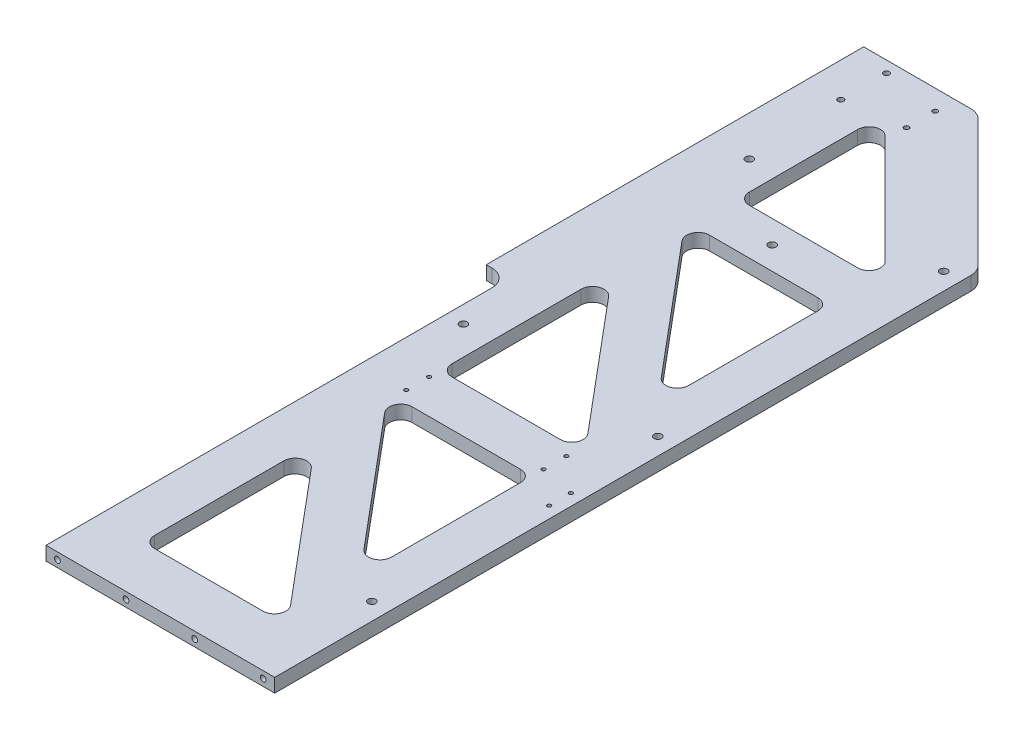
from build123d import *

# Parameters (mm, degrees)
SKETCH_1_W             = 220
SKETCH_1_H             = 330
EXTRUDE_1_DEPTH        = 6
SKETCH_2_W             = 200
SKETCH_2_H             = 405
EXTRUDE_2_DEPTH        = 12
CHAMFER_1_SIZE         = 120
FILLET_2_R             = 15
CUT_EXTRUDE_3_DEPTH    = 12
HOLE_WIZARD_M6_1_D     = 5
HOLE_WIZARD_M6_1_DEPTH = 17
HOLE_WIZARD_M6_1_TIP   = 1.502151548
HOLE_WIZARD_M6_2_D     = 5
HOLE_WIZARD_M6_2_DEPTH = 17
HOLE_WIZARD_M6_2_TIP   = 1.502151548
HOLE_WIZARD_M6_1_2_D   = 6.6
HOLE_WIZARD_M6_2_2_D   = 6.6
HOLE_WIZARD_M6_3_D     = 5
HOLE_WIZARD_M5_1_D     = 4.2
HOLE_WIZARD_M4_1_D     = 3.3
HOLE_WIZARD_M4_2_D     = 3.3


with BuildPart() as part:
    # 草图1 → 凸台-拉伸1 (new, symmetric)
    with BuildSketch(Plane(origin=(0, 0, 0), x_dir=(1, 0, 0), z_dir=(0, 1, 0))):
        Rectangle(SKETCH_1_W, SKETCH_1_H)
    extrude(amount=EXTRUDE_1_DEPTH, both=True)

    # 草图2 → 凸台-拉伸2 (add)
    with BuildSketch(Plane(origin=(0, 6, 0), x_dir=(1, 0, 0), z_dir=(0, 1, 0))):
        with Locations((10, -367.5)):
            Rectangle(SKETCH_2_W, SKETCH_2_H)
    extrude(amount=-EXTRUDE_2_DEPTH)

    # 倒角1
    chamfer_1_edges = [part.edges().sort_by_distance(p)[0] for p in [
        (110, 0, -165),
    ]]
    chamfer(chamfer_1_edges, length=CHAMFER_1_SIZE)

    # 圆角2
    fillet_2_edges = [part.edges().sort_by_distance(p)[0] for p in [
        (-10, 0, -165),
        (110, 0, -45),
        (-90, 0, 165),
    ]]
    fillet(fillet_2_edges, radius=FILLET_2_R)

    # 草图7 → 切除-拉伸3 (cut)
    with BuildSketch(Plane(origin=(0, 6, 0), x_dir=(1, 0, 0), z_dir=(0, 1, 0))):
        with BuildLine():
            Line((-34.747744438, -45), (60, -45))
            ThreePointArc((60, -45), (67.071067812, -47.928932188), (70, -55))
            Line((70, -55), (70, -167.915964824))
            ThreePointArc((70, -167.915964824), (63.420201433, -177.312891032), (52.339555569, -174.343840921))
            Line((52.339555569, -174.343840921), (-42.408188869, -61.427876097))
            ThreePointArc((-42.408188869, -61.427876097), (-43.810822308, -50.773817383), (-34.747744438, -45))
        make_face()
        with BuildLine():
            Line((-32.339555569, -135.656159079), (62.408188869, -248.572123903))
            ThreePointArc((62.408188869, -248.572123903), (63.810822308, -259.226182617), (54.747744438, -265))
            Line((54.747744438, -265), (-40, -265))
            ThreePointArc((-40, -265), (-47.071067812, -262.071067812), (-50, -255))
            Line((-50, -255), (-50, -142.084035176))
            ThreePointArc((-50, -142.084035176), (-43.420201433, -132.687108968), (-32.339555569, -135.656159079))
        make_face()
        with BuildLine():
            Line((-34.747744438, -305), (60, -305))
            ThreePointArc((60, -305), (67.071067812, -307.928932188), (70, -315))
            Line((70, -315), (70, -427.915964824))
            ThreePointArc((70, -427.915964824), (63.420201433, -437.312891032), (52.339555569, -434.343840921))
            Line((52.339555569, -434.343840921), (-42.408188869, -321.427876097))
            ThreePointArc((-42.408188869, -321.427876097), (-43.810822308, -310.773817383), (-34.747744438, -305))
        make_face()
        with BuildLine():
            Line((-32.339555569, -395.656159079), (62.408188869, -508.572123903))
            ThreePointArc((62.408188869, -508.572123903), (63.810822308, -519.226182617), (54.747744438, -525))
            Line((54.747744438, -525), (-40, -525))
            ThreePointArc((-40, -525), (-47.071067812, -522.071067812), (-50, -515))
            Line((-50, -515), (-50, -402.084035176))
            ThreePointArc((-50, -402.084035176), (-43.420201433, -392.687108968), (-32.339555569, -395.656159079))
        make_face()
        with BuildLine():
            Line((-50, 99.747744438), (-50, 5))
            ThreePointArc((-50, 5), (-47.071067812, -2.071067812), (-40, -5))
            Line((-40, -5), (54.747744438, -5))
            ThreePointArc((54.747744438, -5), (63.986539763, 1.173165676), (61.81881225, 12.071067812))
            Line((61.81881225, 12.071067812), (-32.928932188, 106.81881225))
            ThreePointArc((-32.928932188, 106.81881225), (-43.826834324, 108.986539763), (-50, 99.747744438))
        make_face()
    extrude(amount=-CUT_EXTRUDE_3_DEPTH, mode=Mode.SUBTRACT)

    # Hole Wizard M6 _1
    with Locations(Plane.XY.offset(570)):
        with Locations((-80, 0), (-20, 0), (40, 0), (100, 0)):
            Hole(HOLE_WIZARD_M6_1_D / 2, depth=HOLE_WIZARD_M6_1_DEPTH)
            with Locations((0, 0, -(HOLE_WIZARD_M6_1_DEPTH + HOLE_WIZARD_M6_1_TIP / 2))):  # 118° drill point
                Cone(0, HOLE_WIZARD_M6_1_D / 2, HOLE_WIZARD_M6_1_TIP, mode=Mode.SUBTRACT)

    # Hole Wizard M6 _2
    with Locations(Plane.ZY.offset(110)):
        with Locations((-150, 0), (-90, 0), (-30, 0), (30, 0), (90, 0), (150, 0)):
            Hole(HOLE_WIZARD_M6_2_D / 2, depth=HOLE_WIZARD_M6_2_DEPTH)
            with Locations((0, 0, -(HOLE_WIZARD_M6_2_DEPTH + HOLE_WIZARD_M6_2_TIP / 2))):  # 118° drill point
                Cone(0, HOLE_WIZARD_M6_2_D / 2, HOLE_WIZARD_M6_2_TIP, mode=Mode.SUBTRACT)

    # Hole Wizard M6 _1 2 (through all)
    with Locations(Plane(origin=(0, 6, 0), x_dir=(1, 0, 0), z_dir=(0, 1, 0))):
        with Locations((95, 30), (-75, 30), (-75, -220), (95, -220), (95, -470)):
            Hole(HOLE_WIZARD_M6_1_2_D / 2)

    # Hole Wizard M6 _2 2 (through all)
    with Locations(Plane(origin=(0, 6, 0), x_dir=(1, 0, 0), z_dir=(0, 1, 0))):
        with Locations((0, -25)):
            Hole(HOLE_WIZARD_M6_2_2_D / 2)

    # M6 螺纹孔3 (through all)
    with Locations(Plane(origin=(0, 6, 0), x_dir=(1, 0, 0), z_dir=(0, 1, 0))):
        with Locations((-80, 155), (-80, 115)):
            Hole(HOLE_WIZARD_M6_3_D / 2)

    # M5 螺纹孔1 (through all)
    with Locations(Plane(origin=(0, 6, 0), x_dir=(1, 0, 0), z_dir=(0, 1, 0))):
        with Locations((-30, 147.5), (-30, 122.5)):
            Hole(HOLE_WIZARD_M5_1_D / 2)

    # M4 螺纹孔1 (through all)
    with Locations(Plane(origin=(0, 6, 0), x_dir=(1, 0, 0), z_dir=(0, 1, 0))):
        with Locations((100, -320), (100, -301)):
            Hole(HOLE_WIZARD_M4_1_D / 2)

    # M4 螺纹孔2 (through all)
    with Locations(Plane(origin=(0, 6, 0), x_dir=(1, 0, 0), z_dir=(0, 1, 0))):
        with Locations((-50, -275), (70, -275), (70, -295), (-50, -295)):
            Hole(HOLE_WIZARD_M4_2_D / 2)


solid = part.part
